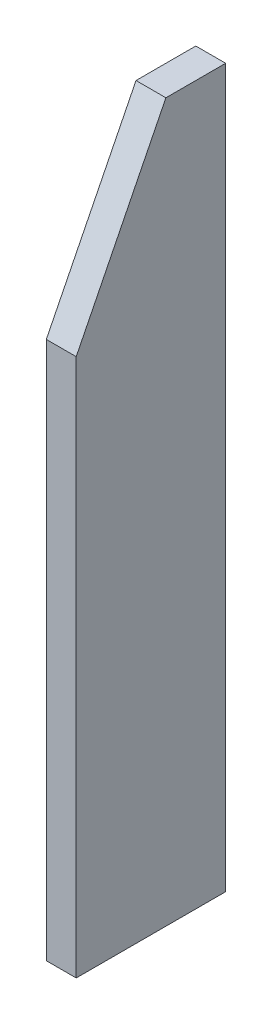
SolidWorks part; units mm, degrees
ref_plane "前视基准面" through (0, 0, 0) normal (0, 0, 1) x (1, 0, 0)
ref_plane "上视基准面" through (0, 0, 0) normal (0, 1, 0) x (1, 0, 0)
ref_plane "右视基准面" through (0, 0, 0) normal (1, 0, 0) x (0, 0, -1)
sketch "草图1" plane through (0, 0, 0) normal (0, 0, 1) x (1, 0, 0)
  line L1 (-5, 120) -> (5, 120)
  line L2 (-5, 120) -> (-5, -120)
  line L3 (-5, -120) -> (5, -120)
  line L4 (5, 120) -> (5, -120)
  line L5 (-5, 120) -> (5, -120) construction
  line L6 (-5, -120) -> (5, 120) construction
  point P0 (0, 0)
  dimension "D1" = 240
  dimension "D2" = 10
extrude "凸台-拉伸1" add sketch "草图1" along normal blind 50
hole_wizard "M4 螺纹孔2" positions "草图10" profile "草图11" tap size "M4" standard "ISO"
sketch "草图10" plane through (0, 0, 0) normal (0, 0, -1) x (-1, 0, 0)
  line L0 (0, 120) -> (0, -120) construction
  line L1 (-5, 120) -> (5, 120) construction
  line L2 (5, -120) -> (-5, -120) construction
  line L3 (-5, 0) -> (5, 0) construction
  line L4 (-5, -120) -> (-5, 120) construction
  line L5 (5, 120) -> (5, -120) construction
  point P0 (0, 97.5)
  point P2 (0, 32.5)
  point P4 (0, -32.5)
  point P6 (0, -97.5)
  dimension "D1" = 65
  dimension "D2" = 65
  dimension "D3" = 65
cosmetic thread "孔螺蚊线1"
cosmetic thread "孔螺蚊线2"
cosmetic thread "孔螺蚊线3"
cosmetic thread "孔螺蚊线4"
sketch "草图11" plane through (0, 97.5, 0) normal (1, 0, 0) x (0, 1, 0)
  line L0 (0, 0) -> (0, 15.9914)
  line L1 (0, 15.9914) -> (1.65, 15)
  line L2 (1.65, 15) -> (1.65, 0)
  line L5 (1.65, 0) -> (0, 0)
  line L10 (0, 15.9914) -> (-1.65, 15) construction
  line L11 (0, -6.35) -> (0, 107.95) construction
  dimension "螺纹孔钻头直径" = 3.3
  dimension "螺纹孔钻头深度" = 15
  dimension "导头角度" = 118
hole_wizard "M4 螺纹孔3" positions "草图12" profile "草图13" tap size "M4" standard "ISO"
sketch "草图12" plane through (0, -120, 0) normal (0, -1, 0) x (-1, 0, 0)
  line L1 (0, -50) -> (0, 0) construction
  line L2 (5, -50) -> (-5, -50) construction
  line L3 (5, 0) -> (-5, 0) construction
  line L5 (5, -25) -> (-5, -25) construction
  line L6 (5, -50) -> (5, 0) construction
  line L7 (-5, -50) -> (-5, 0) construction
  point P0 (0, -10)
  point P2 (0, -40)
  dimension "D1" = 30
sketch "草图13" plane through (0, -120, 10) normal (1, 0, 0) x (0, 0, -1)
  line L0 (0, 0) -> (0, 15.9914)
  line L1 (0, 15.9914) -> (1.65, 15)
  line L2 (1.65, 15) -> (1.65, 0)
  line L5 (1.65, 0) -> (0, 0)
  line L10 (0, 15.9914) -> (-1.65, 15) construction
  line L11 (0, -6.35) -> (0, 107.95) construction
  dimension "螺纹孔钻头直径" = 3.3
  dimension "螺纹孔钻头深度" = 15
  dimension "导头角度" = 118
cosmetic thread "孔螺蚊线5"
cosmetic thread "孔螺蚊线6"
chamfer "倒角1" distance 30 distance2 60 1 edges at (0, 120, 50)
